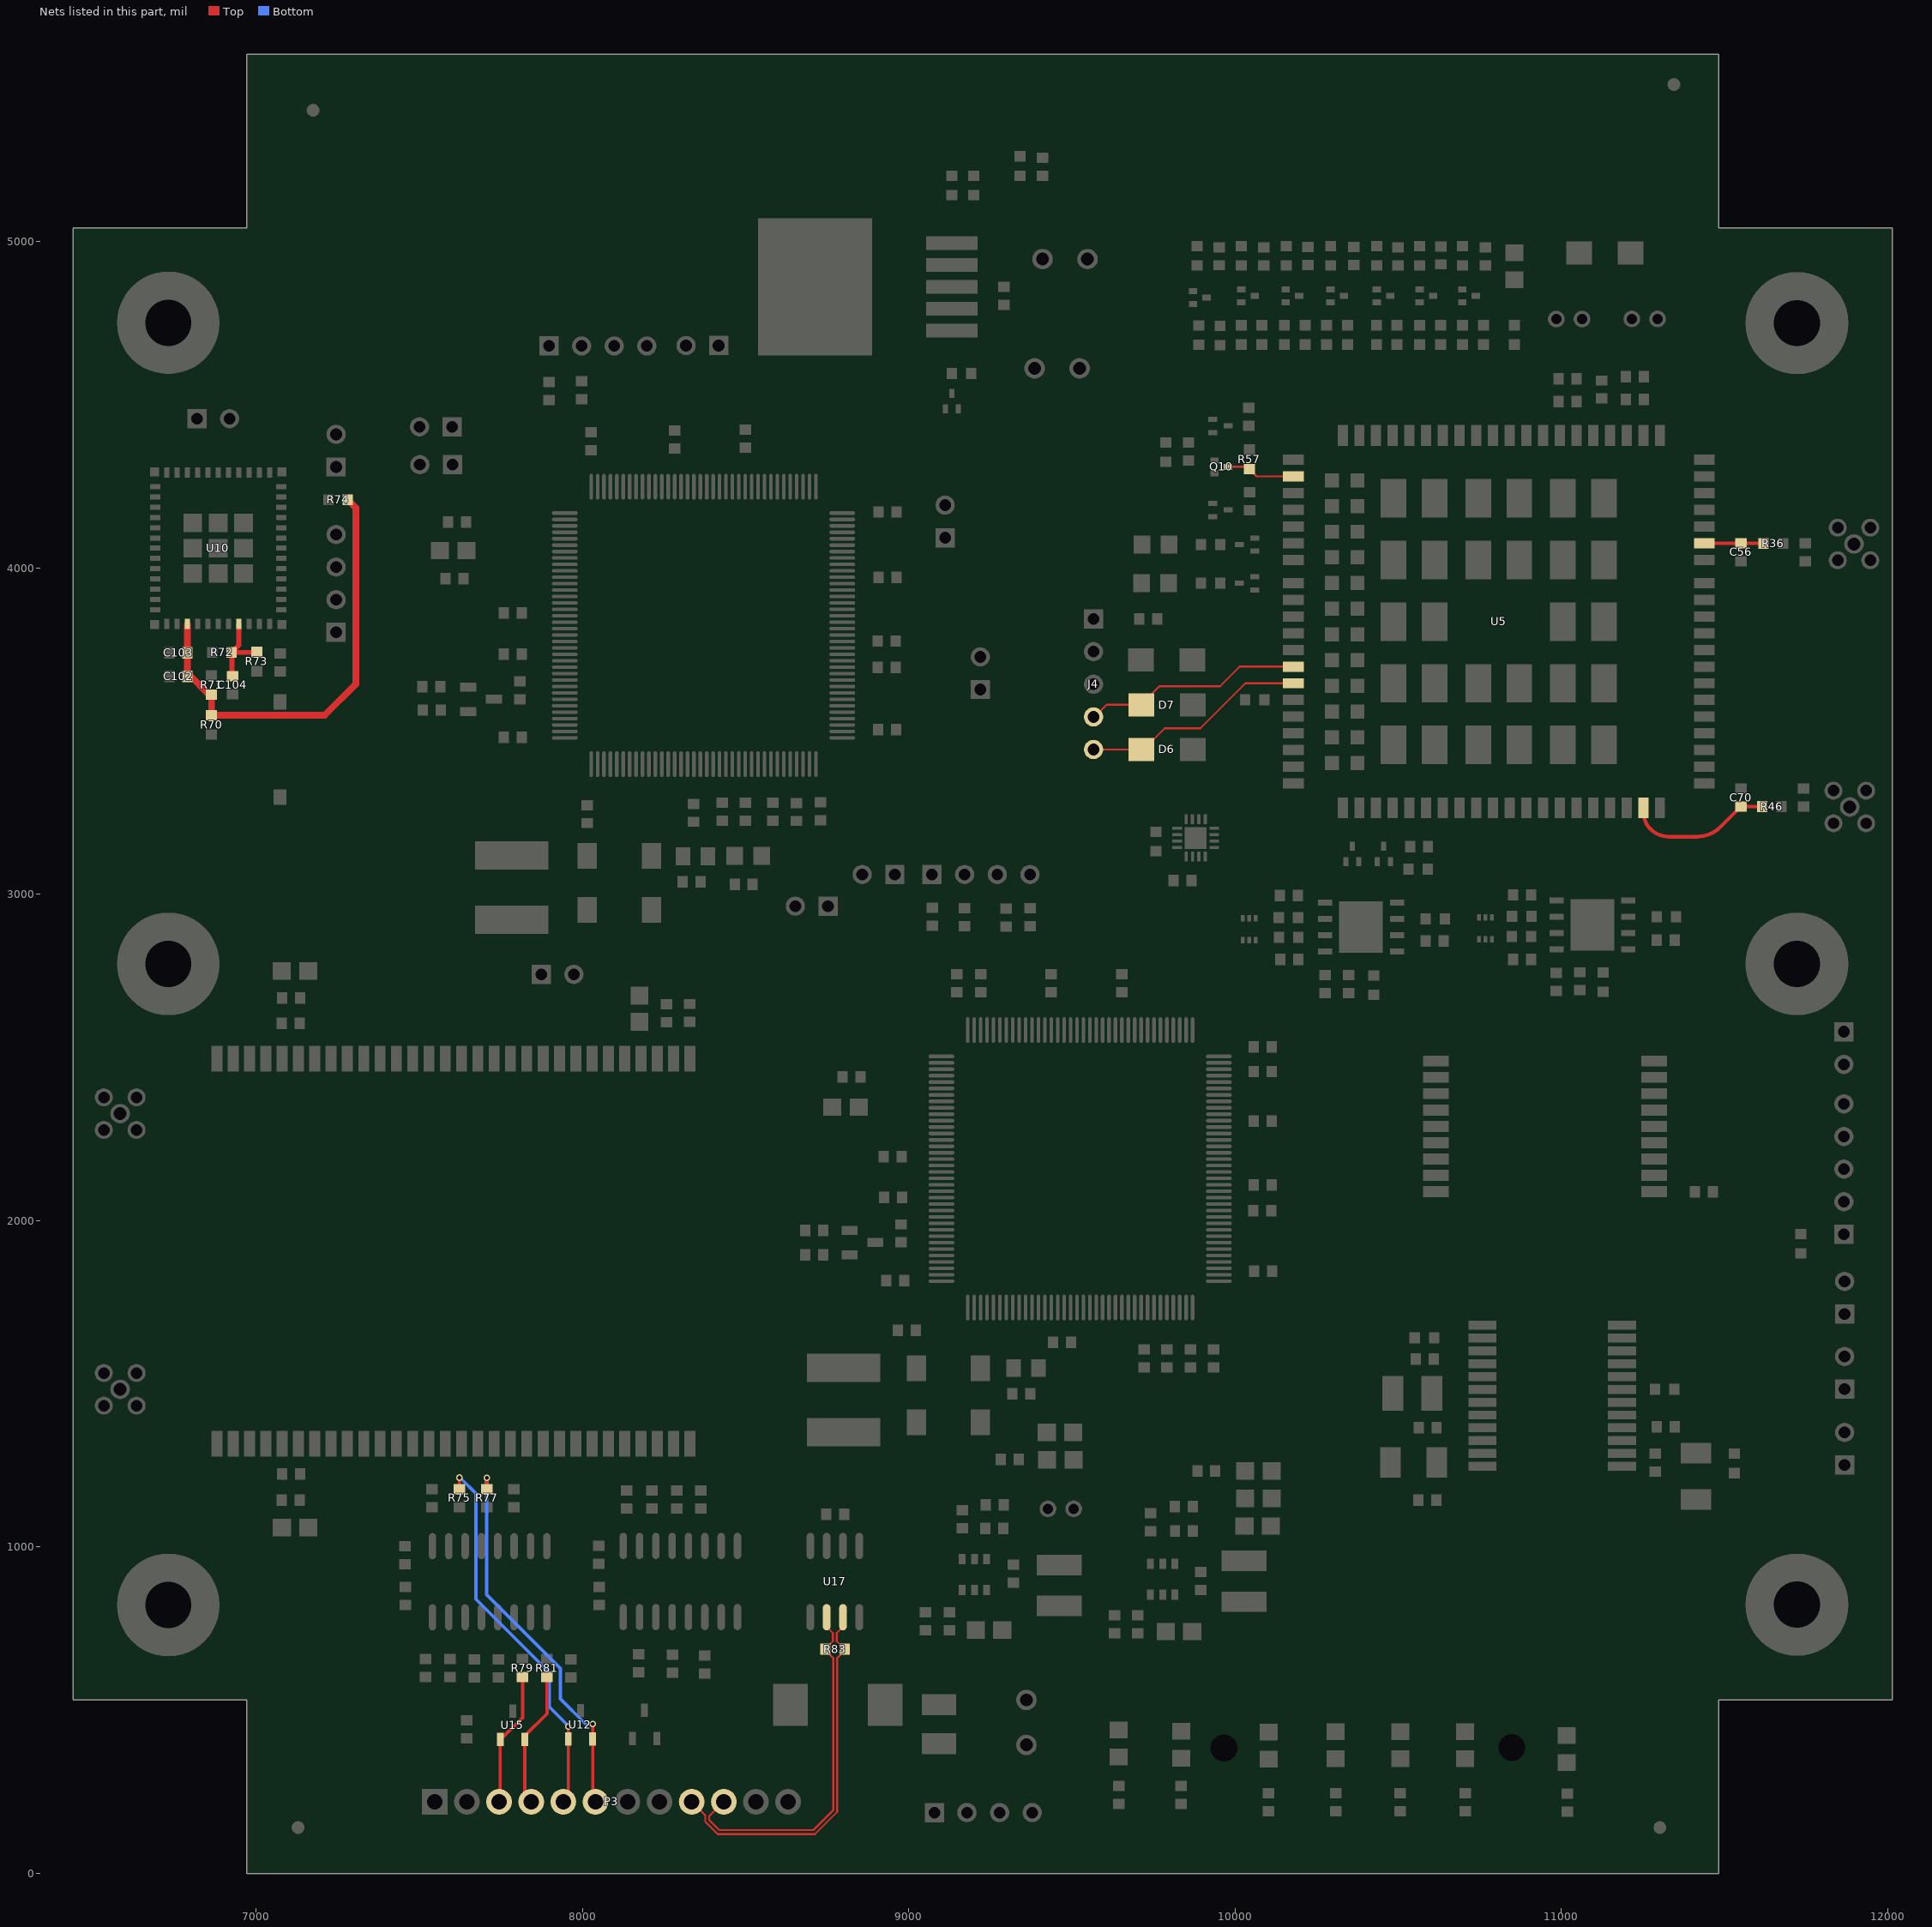
[diagram p0: the nets of this part, all layers, seen from the top]
# Altium PCB MISC86294.PcbDoc (part 3 of 8)
Units mil, origin at the board's own origin, x right, y up, seen from the top; angles counter-clockwise.
Board outline 5574.84 x 5574.84 mil, 4 copper layers (Top, GND02, PWR03, Bottom), stack 23.756 mil thick; 313 components, 311 nets, 1350 pads, 1701 vias.

## Footprints (in the part's own frame and the unit in brackets; to place one, negate y for a bottom-side part, rotate by r counter-clockwise, add the part's x,y. Pads: shape width x height; smd on the part's side, far side on the other; paste and mask are expansions set on the pad) (continued)
SCC2130D [mm]
  rect 0.7x2.2 smd: 1(-5.5,-5.435) 2(-4.5,-5.435) 3(-3.5,-5.435) 4(-2.5,-5.435) 5(-1.5,-5.435) 6(-0.5,-5.435) 7(0.5,-5.435) 8(1.5,-5.435) 9(2.5,-5.435) 10(3.5,-5.435) 11(4.5,-5.435) 12(5.5,-5.435) 13(5.5,5.435) 14(4.5,5.435) 15(3.5,5.435) 16(2.5,5.435) 17(1.5,5.435) 18(0.5,5.435) 19(-0.5,5.435) 20(-1.5,5.435) 21(-2.5,5.435) 22(-3.5,5.435) 23(-4.5,5.435) 24(-5.5,5.435)
  silkscreen extent -7.58,-5.75 7.58,3.75
SMA [mm]
  rect 2x1.8 smd: 1(-2,0) 2(2,0)
  silkscreen extent -2.3,-1.4 2.3,1.4
SMC_L6.9-W5.9-LS7.9-RD [mm]
  rect 2.7x3.3 smd: 1(-3.686,0) 2(3.686,0)
  silkscreen extent -4.36,-3.1 3.98,3.1
SMD [mm]
  rect 1.2x1 smd: 1(-3.7,0) 2(3.7,0)
  silkscreen extent -3.05,-1.8 3.05,1.8
SMD_L6.0-W6.0 [mm]
  rect 2.2x5.72 smd: 1(-2.5,0) 2(2.5,0)
  silkscreen extent -3.18,-3.18 3.18,3.18
SOIC-8 [mm]
  oval 0.588x2.045 smd: 1(-2.535,-1.748) 2(-1.265,-1.748) 3(0.005,-1.748) 4(1.275,-1.748) 5(1.275,3.797) 6(0.005,3.797) 7(-1.265,3.797) 8(-2.535,3.797)
  silkscreen extent -3.43,-1.9 1.9,2.55
SOP16-6_6 [mil]
  oval 22.6x80.24 smd: 1(-170.43,-109.02) 2(-120.43,-109.02) 3(-70.43,-109.02) 4(-20.43,-109.02) 5(29.57,-109.02) 6(79.57,-109.02) 7(129.57,-109.02) 8(179.57,-109.02) 9(179.57,109.02) 10(129.57,109.02) 11(79.57,109.02) 12(29.57,109.02) 13(-20.43,109.02) 14(-70.43,109.02) 15(-120.43,109.02) 16(-170.43,109.02)
  silkscreen extent -205,-115 202,60
SOT-23 [mil]
  rect 40.85x20.95 smd: 1(136.15,-108.1) 2(136.15,-33.3) 3(49.44,-70.7)
  silkscreen extent 59,-131 127,-11
SOT-23-SS8550 [mm]
  rect 1.25x0.7 smd: 1(1,-0.95) 2(1,0.95) 3(-1,0)
  silkscreen extent -0.73,-1.53 0.73,1.53
SOT-416_L1_6-W0_8-P1_00-LS1_6-BR [mm]
  rect 0.7x0.4 smd: 1(0.563,-0.508) 2(0.563,0.508) 3(-0.637,0)
  silkscreen extent -0.44,-0.85 0.36,0.85
SOT-563 [mm]
  rect 0.5x0.3 smd: 1(0.85,-0.424) 2(0.85,0.076) 3(0.85,0.576) 4(-0.85,0.576) 5(-0.85,0.076) 6(-0.85,-0.424)
  silkscreen extent -0.48,-0.91 0.9,0.86
TO-263-5 [mm]
  rect 4x1.069 smd: 1(-6.556,3.4) 2(-6.556,1.7) 3(-6.556,0) 4(-6.556,-1.7) 5(-6.556,-3.4)
  rect 8.89x10.66 smd: 6(4.111,0)
  silkscreen extent -4.27,-5.1 -0.56,5.1
TQFN-16_L3.0-W3.0-P0.50-BL-EP1.7 [mm]
  rect 0.25x0.75 smd: 1(-0.748,-1.275) 2(-0.249,-1.275) 3(0.252,-1.275) 4(0.751,-1.275) 9(0.75,1.625) 10(0.25,1.625) 11(-0.25,1.625) 12(-0.749,1.625)
  rect 0.75x0.25 smd: 5(1.45,-0.575) 6(1.45,-0.075) 7(1.45,0.425) 8(1.45,0.925) 13(-1.45,0.925) 14(-1.45,0.425) 15(-1.45,-0.075) 16(-1.45,-0.575)
  rect 1.7x1.7 smd: 17(0,0.175)
  silkscreen extent -1.5,-2 1.5,1.68
TSOT-23-6_L2.9-W1.6-P0.95-LS2.8-BR [mm]
  rect 0.8x0.532 smd: 1(1.2,-0.95) 2(1.2,0) 3(1.2,0.95) 4(-1.2,0.95) 5(-1.2,0) 6(-1.2,-0.95)
  silkscreen extent -0.88,-1.82 1.44,1.53
UM482_K823 [mm]
  rect 2.01x0.85 smd: 1(-14.903,18.415) 2(-14.903,17.145) 3(-14.903,15.875) 4(-14.903,14.605) 5(-14.903,13.335) 6(-14.903,12.065) 7(-14.903,10.795) 8(-14.903,9.525) 9(-14.903,8.255) 10(-14.903,6.985) 11(-14.903,5.715) 12(-14.903,4.445) 13(-14.903,3.175) 14(-14.903,1.905) 15(-14.903,0.635) 16(-14.903,-0.635) 17(-14.903,-1.905) 18(-14.903,-3.175) 19(-14.903,-4.445) 20(-14.903,-5.715) 21(-14.903,-6.985) 22(-14.903,-8.255) 23(-14.903,-9.525) 24(-14.903,-10.795) 25(-14.903,-12.065) 26(-14.903,-13.335) 27(-14.903,-14.605) 28(-14.903,-15.875) 29(-14.903,-17.145) 30(-14.903,-18.415) 31(15.097,-18.415) 32(15.097,-17.145) 33(15.097,-15.875) 34(15.097,-14.605) 35(15.097,-13.335) 36(15.097,-12.065) 37(15.097,-10.795) 38(15.097,-9.525) 39(15.097,-8.255) 40(15.097,-6.985) 41(15.097,-5.715) 42(15.097,-4.445) 43(15.097,-3.175) 44(15.097,-1.905) 45(15.097,-0.635) 46(15.097,0.635) 47(15.097,1.905) 48(15.097,3.175) 49(15.097,4.445) 50(15.097,5.715) 51(15.097,6.985) 52(15.097,8.255) 53(15.097,9.525) 54(15.097,10.795) 55(15.097,12.065) 56(15.097,13.335) 57(15.097,14.605) 58(15.097,15.875) 59(15.097,17.145) 60(15.097,18.415)
  silkscreen extent -16.1,-20 15.1,20
WIFIM-SMD_ESP32-C3-MINI-1 [mm]
  rect 0.8x0.4 smd: 1(-5.9,4) 2(-5.9,3.2) 3(-5.9,2.4) 4(-5.9,1.6) 5(-5.9,0.8) 6(-5.9,0) 7(-5.9,-0.8) 8(-5.9,-1.6) 9(-5.9,-2.4) 10(-5.9,-3.2) 11(-5.9,-4) 25(5.9,-4) 26(5.9,-3.2) 27(5.9,-2.4) 28(5.9,-1.6) 29(5.9,-0.8) 30(5.9,0) 31(5.9,0.8) 32(5.9,1.6) 33(5.9,2.4) 34(5.9,3.2) 35(5.9,4)
  rect 0.4x0.8 smd: 12(-4.8,-4.9) 13(-4,-4.9) 14(-3.2,-4.9) 15(-2.4,-4.9) 16(-1.6,-4.9) 17(-0.8,-4.9) 18(0,-4.9) 19(0.8,-4.9) 20(1.6,-4.9) 21(2.4,-4.9) 22(3.2,-4.9) 23(4,-4.9) 24(4.8,-4.9) 36(4.8,4.9) 37(4,4.9) 38(3.2,4.9) 39(2.4,4.9) 40(1.6,4.9) 41(0.8,4.9) 42(0,4.9) 43(-0.8,4.9) 44(-1.6,4.9) 45(-2.4,4.9) 46(-3.2,4.9) 47(-4,4.9) 48(-4.8,4.9)
  rect 1.45x1.45 smd: 49(-1.975,-1.975) 49(-1.975,0) 49(-1.975,1.975) 49(0,1.975) 49(0,0) 49(0,-1.975) 49(1.975,-1.975) 49(1.975,0) 49(1.975,1.975)
  rect 0.7x0.7 smd: 50(5.95,4.95) 51(5.95,-4.95) 52(-5.95,-4.95) 53(-5.95,4.95)
  silkscreen extent -7.1,-5.6 6.6,11
XH-12A [mm]
  rect 2x2 hole 1.2: 1(-13.75,0)
  round 2 hole 1.2: 2(-11.25,0) 3(-8.75,0) 4(-6.25,0) 5(-3.75,0) 6(-1.25,0) 7(1.25,0) 8(3.75,0) 9(6.25,0) 10(8.75,0) 11(11.25,0) 12(13.75,0)
  silkscreen extent -16.25,-2.3 16.25,3.5
"XTAL 5.7X7.0-SM - duplicate" [mm]
  rect 1.5x2 smd: 1(-2.5,-2.1) 2(2.5,-2.1) 3(2.5,2.1) 4(-2.5,2.1)
  silkscreen extent -4.5,-2.65 3.7,2.65, body extent -3.55,-2.55 3.45,2.45, height 1.5

## Part data
C1 C19: library part Cap_C14
C2 C3 C4 C5 C6 C7 C8 C9 C10 C11 C12 C13 C14 C15 C16 C17 C18 C20 C21 C22 C23 C24 C25 C26 C27 C28 C29 C30 C31 C32 C33 C34: library part "CAP NP_Dup1"
C35 C100: library part Cap_C17
C36 C37: library part Cap_C2
C38 C39 C41 C45 C122: library part Cap, "SMD ceramic capacitor"
C40 C42: library part Cap, "SMD ceramic capacitor, X5R"
C43: library part Cap2, "100μF,10V,Φ5×7mm,RoHS"
C44: library part Cap, "SMD ceramic capacitor, MLCC"
C46: library part Cap, "470μF,25V,Φ8×11.5mm,RoHS"
C47 C48 C49 C50 C51 C53 C92: library part Cap, "Capacitor"
C52: library part Cap2, "Capacitor"
C54: library part Cap_C54
C55: library part Cap_C97
C56: library part Cap_C98
C57: library part Cap_C109
C58: library part Cap_C113
C59: library part Cap2_C77
C60: library part Cap_C73
C61: library part Cap_C74
C62: library part Cap_C75
C63: library part Cap_C114
C64: library part Cap2_C76
C65: library part Cap_C70
C66: library part Cap_C71
C67: library part Cap_C72
C68: library part Cap_C115
C69: library part Cap_C102
C70: library part Cap_C103
C71: library part Cap_C116
C72: library part Cap_C117
C73: library part Cap_C58
C74: library part Cap_C91
C75: library part Cap_C101
C76: library part Cap_C104
C77: library part Cap_C105
C78: library part Cap_C48_Dup1
C79: library part Cap_C32_Dup1
C80 C93: library part Cap_C45_Dup1
C81: library part Cap_C47_Dup1
C82 C123: library part Cap_C51_Dup1
C83 C128: library part Cap_C49_Dup1
C84 C129: library part Cap_C50
C85 C130: library part Cap_C52_Dup1
C86: library part Cap_C3
C87: library part Cap_C5
C88: library part Cap_C6
C89: library part Cap_C7
C90: library part Cap_C8
C91: library part Cap_C4
C94: library part Cap_C9
C95: library part Cap_C10
C96: library part Cap_C13
C97: library part Cap_C11
C98: library part Cap_C12
C99: library part Cap_C16
C101: library part Cap_C15
C102 C103 C104 C105: library part Cap_C90
C106: library part Cap_C18
C107: library part Cap_C19
C108: library part Cap_C21
C109: library part Cap_C36
C110: library part Cap_C20
C111: library part Cap_C37
C112: library part Cap_C38
C113: library part Cap_C24
C114: library part Cap_C39
C115: library part Cap_C22
C116: library part Cap_C23
C117: library part Cap_C42
C118: library part Cap_C40
C119: library part Cap_C41
C120: library part Cap_C26
C121: library part Cap_C27
C124: library part Cap_C106
C200 C201 C202 C203: library part Cap, "SMD capacitor"
D1: library part Diode, "TVS diode"
D2: library part LED1, "Red high-brightness LED"
D3 D11 D12 D13 D14 D15 D16: library part LED1_D4
D4: library part Diode_1_D8
D5: library part Diode_1_D14
D6: library part Diode_1_D15
D7: library part Diode_1_D16
D8: library part LED1_D21
D9: library part LED1_D22
D10: library part LED1_D23
J2: library part CIRCLE_J19
J3: library part CIRCLE_J21
J5: library part CIRCLE_J1
J6: library part UM482_J2
J7: library part CIRCLE_J3
J8: library part "HEADER 4"
J9 J10 J12 J13 J14 J15 J16 J17 J18 J19 J20 J21 J22 J23: library part "HEADER 2"
J11: library part 2.54_J4
L1 L4: library part Inductor, "SMD power inductor, cjiang (Changjiang Micro), FNR4026S2R2MT"
L2: library part Inductor_L1
L3: library part Inductor, "Ferrite bead"
L200 L201: library part Inductor, "SMD inductor"
P1 P2: library part "Header 4_P1"
P3: library part "HEADER 12"
Q1 Q2: library part PNP_Q1
Q11: library part DTC043ZEBTL_Q10
Q12: library part DTC043ZEBTL_Q6
Q13: library part DTC043ZEBTL_Q4
Q14: library part DTC043ZEBTL_Q3
Q15: library part DTC043ZEBTL_Q12
Q16: library part DTC043ZEBTL_Q13
Q17: library part DTC043ZEBTL_Q5
R1 R13: library part Res_R2
R2 R14: library part Res_R3
R3 R16: library part Res_R4
R4 R15: library part Res_R5
R5 R18: library part Res_R1
R6 R84 R92 R93: library part Res1_R8
R7: library part Res1_R10
R8 R10 R17 R19: library part Res1_R21
R9 R98: library part Res1_R12
R11 R20: library part Res1_R6
R12 R21: library part Res1_R7
R22 R23 R24 R25 R70 R71 R72 R73 R74: library part Res1_R57
R26 R27 R28 R30 R31 R32 R33: library part Res1, "SMD resistor"
R29: library part RES, "Resettable fuse"
R34: library part Res1_R99
R35: library part Res1_R100
R36: library part Res1_R62
R37: library part Res1_R101
R38: library part Res1_R102
R39: library part Res1_R103
R40: library part Res1_R104
R41: library part Res1_R26_Dup1
R42: library part Res1_R105
R43: library part Res1_R106
R44: library part Res1_R108
R45: library part Res1_R107
R46: library part Res1_R64
R47: library part Res1_R109
R48: library part Res1_R27_Dup1
R49: library part Res1_R110
R50: library part Res1_R111
R51: library part Res1_R28_Dup1
R52: library part Res1_R112
R53: library part Res1_R32
R54: library part Res1_R113
R55 R85: library part Res1_R114
R56: library part Res1_R115
R57: library part Res1_R30
R58: library part Res1_R31
R59: library part Res1_R65
R60: library part Res1_R66
R61: library part Res1_R67
R62: library part Res1_R42
R63: library part Res1_R68
R64: library part Res1_R78
R65: library part Res1_R79
R66: library part Res1_R80
R67 R82: library part Res1_R23
R68 R80 R86 R87: library part Res1_R21_Dup1
R69 R90: library part Res1_R24
R75: library part RES_R14
R76: library part RES_R22
R77: library part RES_R16
R78: library part RES_R23
R79: library part RES_R17
R81: library part RES_R18
R83: library part Res1_R90
R91: library part Res1, "Resistor"
R200 R201: library part Res, "SMD resistor"
SW1: library part SW_PB_SPST
U3: library part FSS-IMU614-AG
U6: library part MIC29302WU_U22
U7 U19: library part SIM-A_U25
U8 U21: library part ESDA6V8V6-6_U26
U9: library part SCC2130_U2
U11: library part SP202ECT_U3
U12: library part PESD12VL2BT_U4
U13: library part PESD12VL2BT_U8
U14: library part SP202ECT_U7
U15: library part PESD12VL2BT_U5
U17: library part TJA1040T_U18
U20: library part FSA2567
Y1 Y2: library part "Header 2X2", "Header, 2-Pin, Dual row"

## Free pads (board coordinates)
  round 314.96 hole 141.73: 0(6730,822) 0(6730,2787) 0(6730,4752) 0(11722,823) 0(11722,2787) 0(11722,4751)
  round 40 hole 82.68 slot 122.05 at 90 deg unplated: 1(9966,384) 1(10848,385)
  round 39.37 smd mask+39.37: MARK(7128,140) MARK(7174,5403) MARK(11302,140) MARK(11345,5482)

## Via types
v1: diameter 20, hole 12, Top to Bottom, 1701 vias

## Nets (pads, with @x,y where several pads share a name; then routed paths per layer and width w, separated by ;. In a path a pad name is that pad's centre, name@x,y a point inside that pad or via, vN(x,y) a via of type N, cw(c..) or ccw(c..) an arc to the next point about the centre after c; other vN are vias at no path point)
232RX0: P3.6 R77.1 U12.2 | length 1145.7
  Top w10: R77.1@7706.14,1177.45 v1(7706.14,1212.14) ; P3.6@8031,234 U12.2@8031,412 ; U12.2@8031,426 v1(8031,457)
  Bottom w10: v1(7706.14,1212.14) 7706.14,853.86 7932,628 7932,534 8010,456 v1@8030,456
232RX1: P3.4 R81.1 U15.2 | length 406.2
  Top w10: P3.4@7838,229 7823,244 7823,421 7890.81,488.81 R81.1@7890.81,600.85
232TX0: P3.5 R75.1 U12.1 | length 1144.9
  Top w10: R75.1@7622.39,1177.45 v1(7622.39,1212.39) ; P3.5@7956.2,239.2 U12.1@7956.2,412 v1(7956.2,449.8)
  Bottom w10: v1@7625,1212 7673,1164 7673,840 7898,615 7898,510 v1@7956,452 ; v1(7956.2,449.8) v1@7956.2,452
232TX1: P3.3 R79.1 U15.1 | length 394.8
  Top w10: P3.3@7746,235 7747,236 7747,408 7815.92,476.92 R79.1@7815.92,600.85
ANT_DIV: C70.2 R46.1 U5.35 | length 456.9
  Top w11.55: U5.35@11253,3264 11253,3246.87 ccw(c11317.87,3246.87) 11272,3201 ccw(c11329.94,3258.94) 11329.94,3177 11330,3177 11416.33,3177 ccw(c11416.33,3277) 11487.04,3206.29 C70.2@11549.83,3269.07 ; C70.2@11544.93,3269.07 C70.2@11549.83,3269.07 ; C70.2@11549.89,3269.14 C70.2@11549.83,3269.07 ; R46.1@11615.58,3269.07 C70.2@11549.83,3269.07
ANT_MAIN: C56.2 R36.1 U5.49 | length 182.9
  Top w11.55: U5.49@11437.92,4076.16 R36.1@11620.83,4076.16
AP_READY_MODULE: Q10.3 R57.2 U5.2 | length 209.6
  Top w6: Q10.3@9981,4311 10036,4311 10066.11,4280.89 U5.2@10178.08,4280.89
CANH: P3.9 R83.1 U17.7 | length 1137.7
  Top w6: P3.9@8334.43,219.05 8376,177.49 8376,158.03 8414.03,120 8712,120 8780,188 8780,659 8801,680 R83.1@8800,680 ; U17.7@8798,784.7 8798,755 8779,736 8779,711 R83.1@8799,691
CANL: P3.10 R83.2 U17.6 | length 1098.4
  Top w6: P3.10@8432.86,219.05 8432.05,219.05 8388,175 8388,163 8419,132 8707.03,132 8768,192.97 8768,660 R83.2@8748,680 ; R83.2@8747,691 8767,711 8767,736 8748,755 U17.6@8748,784.7
DBG_RXD: D7.2 J4.4 U5.11 | length 657.4
  Top w6: J4.4@9580,3555 9606,3581 9711,3581 9768,3638 9954,3638 10014.2,3698.2 U5.11@10178.08,3698.2
DBG_TXD: D6.2 J4.5 U5.12 | length 683.2
  Top w6: J4.5@9579,3444 9719,3444 9784,3509 9893,3509 10031.02,3647.02 U5.12@10178.08,3647.02
EN: C104.2 R72.2 R73.1 U10.8 | length 234.8
  Top w15: R72.2@6924.19,3741.57 R72.2@6925,3741.57 ; C104.2@6925,3674 R72.2@6925,3741.57 ; U10.8@6945.99,3828.72 6945.99,3763.99 6925,3743 R72.2@6925,3741.57 ; R73.1@6995.57,3741.57 R72.2@6925,3741.57
ESP_VCC: C102.2 C103.2 R70.2 R71.2 R74.1 U10.3 | length 1378.9
  Top w20: C102.2@6788.51,3679 U10.3@6788.51,3828.72 ; C102.2@6790,3679 6790,3677 6855.12,3611.88 R71.2@6862.43,3611.88 R70.2@6862.43,3551.57 ; R70.2@6862.43,3549.19 7210.19,3549.19 7305,3644 7305,3690 ; R74.1@7280.27,4209.43 7305,4184.7 7305,3690 ; 7305,3680 7305,3690